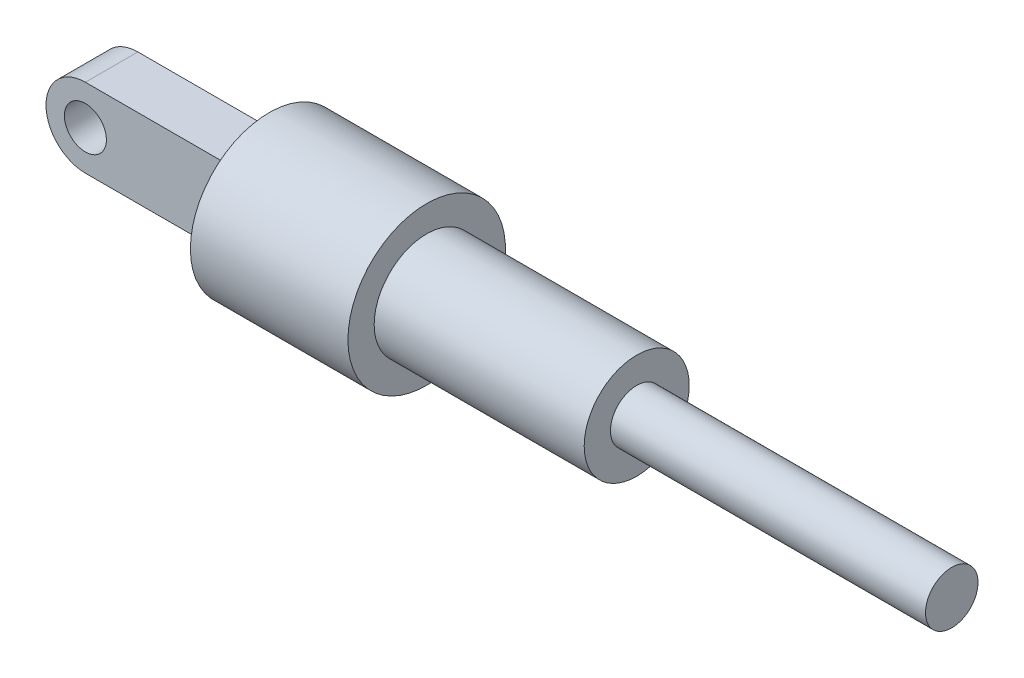
from build123d import *

# Parameters (mm, degrees)
SKETCH2_R           = 0.4
BOSS_EXTRUDE1_DEPTH = 0.5
SKETCH4_R           = 1
SKETCH4_R_2         = 0.5
CUT_EXTRUDE3_DEPTH  = 6


with BuildPart() as part:
    # Sketch1 → Revolve1 (revolve)
    with BuildSketch(Plane.XY, mode=Mode.PRIVATE) as revolve1_sk:
        Polygon((0, 0), (0, 1.5), (3, 1.5), (3, 1), (13, 1), (13, 0), align=None)
    revolve(revolve1_sk.sketch.rotate(Axis((0.124352332, 0, 0), (1, 0, 0)), 90), axis=Axis((0.124352332, 0, 0), (1, 0, 0)))

    # Sketch2 → Boss-Extrude1 (add, symmetric)
    with BuildSketch(Plane.XY):
        with BuildLine():
            Line((0, 0.75), (0, -0.75))
            Line((0, -0.75), (-3, -0.75))
            ThreePointArc((-3, -0.75), (-3.75, 0), (-3, 0.75))
            Line((-3, 0.75), (0, 0.75))
        make_face()
        with Locations((-3, 0)):
            Circle(SKETCH2_R, mode=Mode.SUBTRACT)
    extrude(amount=BOSS_EXTRUDE1_DEPTH, both=True)

    # Sketch4 → Cut-Extrude3 (cut)
    with BuildSketch(Plane(origin=(13, 0, 0), x_dir=(0, 0, -1), z_dir=(1, 0, 0))):
        with Locations(Location((0, 0, 0), (0, 0, 180))):
            Circle(SKETCH4_R)
        Circle(SKETCH4_R_2, mode=Mode.SUBTRACT)
    extrude(amount=-CUT_EXTRUDE3_DEPTH, mode=Mode.SUBTRACT)


solid = part.part
